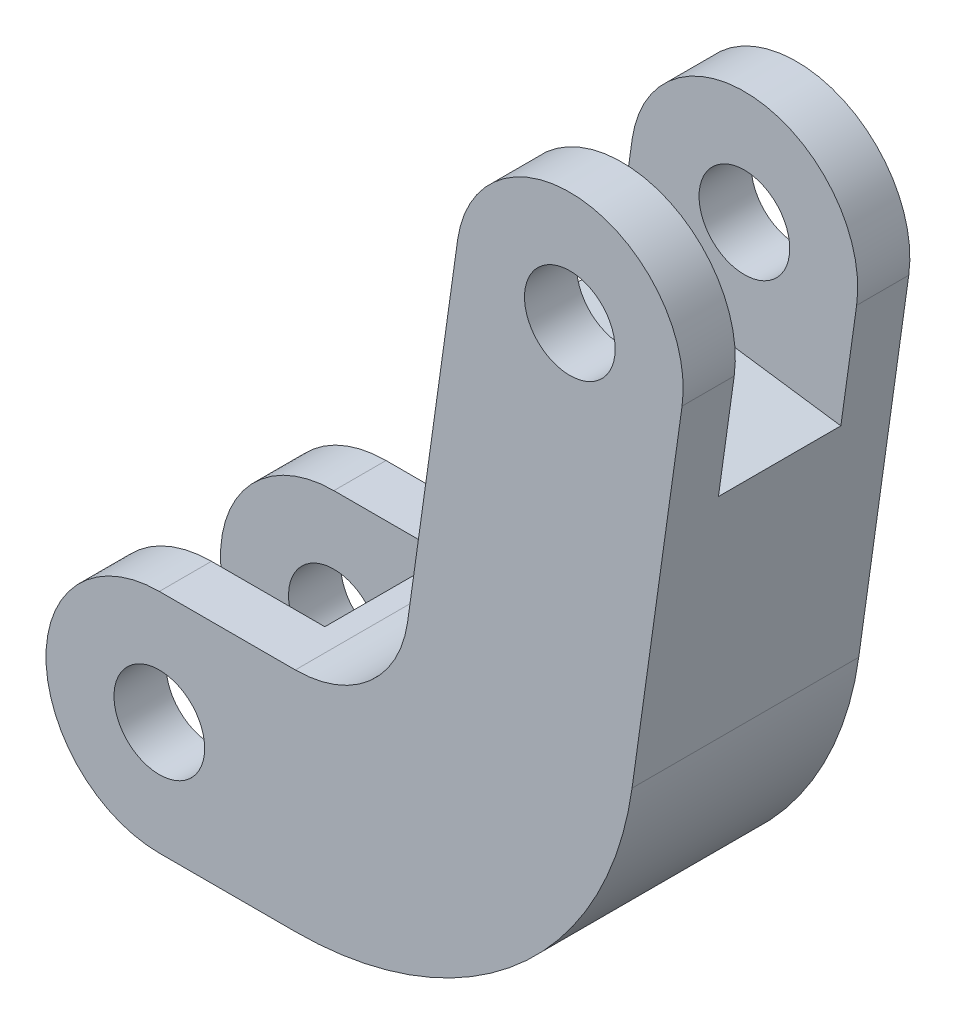
from build123d import *

# Parameters (mm, degrees)
BOSS_EXTRUDE1_DEPTH     = 5
CUT_EXTRUDE1_DEPTH      = 34.907195681
CUT_EXTRUDE1_DEPTH_BACK = 34.907195681
SKETCH2_R               = 2
SKETCH3_W               = 5.4
SKETCH3_H               = 10
CUT_EXTRUDE2_DEPTH      = 10
SKETCH4_R               = 2
CUT_EXTRUDE3_DEPTH      = 31
SKETCH7_W               = 5.4
SKETCH7_H               = 10
CUT_EXTRUDE5_DEPTH      = 13


with BuildPart() as part:
    # Sketch1 → Boss-Extrude1 (new, symmetric)
    with BuildSketch(Plane.XY):
        with BuildLine():
            Line((10.951340344, 4.304134495), (13.157250383, 20))
            ThreePointArc((13.157250383, 20), (18.804456232, 24.255474839), (23.059931071, 18.60826899))
            Line((23.059931071, 18.60826899), (20.854021031, 2.912403486))
            ThreePointArc((20.854021031, 2.912403486), (15.840885435, -6.320643703), (6, -10))
            Line((6, -10), (0, -10))
            ThreePointArc((0, -10), (-5, -5), (0, 0))
            Line((0, 0), (6, 0))
            ThreePointArc((6, 0), (9.280295145, 1.226452099), (10.951340344, 4.304134495))
        make_face()
    extrude(amount=BOSS_EXTRUDE1_DEPTH, both=True)

    # Sketch2 → Cut-Extrude1 (cut, two sides: drawn at the far end of the back side and taken through both)
    with BuildSketch(Plane.XY.offset(-CUT_EXTRUDE1_DEPTH_BACK)):
        with Locations((0, -5)):
            Circle(SKETCH2_R)
    extrude(amount=CUT_EXTRUDE1_DEPTH + CUT_EXTRUDE1_DEPTH_BACK, mode=Mode.SUBTRACT)

    # Sketch3 → Cut-Extrude2 (cut)
    with BuildSketch(Plane(origin=(-5, 0, 0), x_dir=(0, 0, -1), z_dir=(1, 0, 0))):
        with Locations((0, -5)):
            Rectangle(SKETCH3_W, SKETCH3_H)
    extrude(amount=CUT_EXTRUDE2_DEPTH, mode=Mode.SUBTRACT)

    # Sketch4 → Cut-Extrude3 (cut)
    with BuildSketch(Plane.XY.offset(5)):
        with Locations((18.108590727, 19.304134495)):
            Circle(SKETCH4_R)
    extrude(amount=-CUT_EXTRUDE3_DEPTH, mode=Mode.SUBTRACT)

    # Sketch7 → Cut-Extrude5 (cut)
    with BuildSketch(Plane(origin=(20.048712729, -2.817662822, 0), x_dir=(0, 0, -1), z_dir=(0.9902680687415704, -0.13917310096006613, 0))):
        with Locations((0, 21.636496711)):
            Rectangle(SKETCH7_W, SKETCH7_H)
    extrude(amount=-CUT_EXTRUDE5_DEPTH, mode=Mode.SUBTRACT)


solid = part.part
